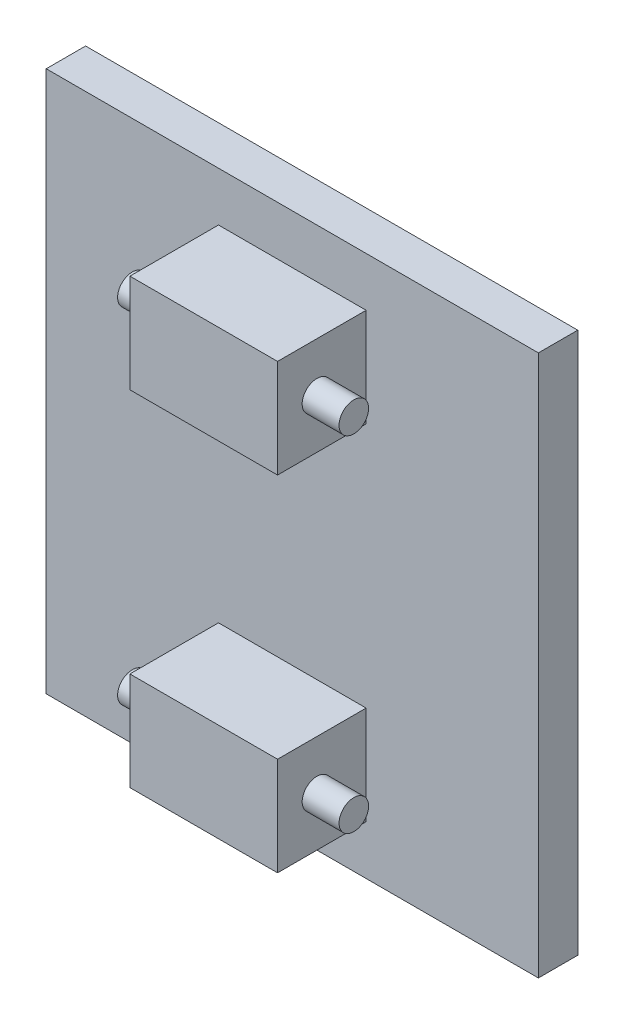
from build123d import *

# Parameters (mm, degrees)
SKETCH1_W           = 100
SKETCH1_H           = 110
BOSS_EXTRUDE1_DEPTH = 8
SKETCH2_W           = 30
SKETCH2_H           = 20
BOSS_EXTRUDE2_DEPTH = 18
SKETCH4_W           = 29.345369705
SKETCH4_H           = 91.568125834
SKETCH4_W_2         = 32.679168461
SKETCH4_H_2         = 92.103849907
CUT_EXTRUDE2_DEPTH  = 5
SKETCH3_R           = 3
BOSS_EXTRUDE3_DEPTH = 22.5


with BuildPart() as part:
    # Sketch1 → Boss-Extrude1 (new body)
    with BuildSketch(Plane.XY):
        Rectangle(SKETCH1_W, SKETCH1_H)
    extrude(amount=BOSS_EXTRUDE1_DEPTH)

    # Sketch2 → Boss-Extrude2 (add)
    with BuildSketch(Plane.XY.offset(8)):
        with Locations((0, 35)):
            Rectangle(SKETCH2_W, SKETCH2_H)
        with Locations((0, -35)):
            Rectangle(SKETCH2_W, SKETCH2_H)
    extrude(amount=BOSS_EXTRUDE2_DEPTH)

    # Sketch4 → Cut-Extrude2 (cut)
    with BuildSketch(Plane(origin=(0, 0, 0), x_dir=(-1, 0, 0), z_dir=(0, 0, -1))):
        with Locations((-27.976499336, 2.033263611)):
            Rectangle(SKETCH4_W, SKETCH4_H)
        with Locations((27.679077111, 1.765401575)):
            Rectangle(SKETCH4_W_2, SKETCH4_H_2)
    extrude(amount=-CUT_EXTRUDE2_DEPTH, mode=Mode.SUBTRACT)

    # Sketch3 → Boss-Extrude3 (add, symmetric)
    with BuildSketch(Plane(origin=(0, 0, 0), x_dir=(0, 0, -1), z_dir=(1, 0, 0))):
        with Locations(Location((-18, 35, 0), (0, 0, 180))):
            Circle(SKETCH3_R)
        with Locations(Location((-18, -35, 0), (0, 0, 180))):
            Circle(SKETCH3_R)
    extrude(amount=BOSS_EXTRUDE3_DEPTH, both=True)


solid = part.part
